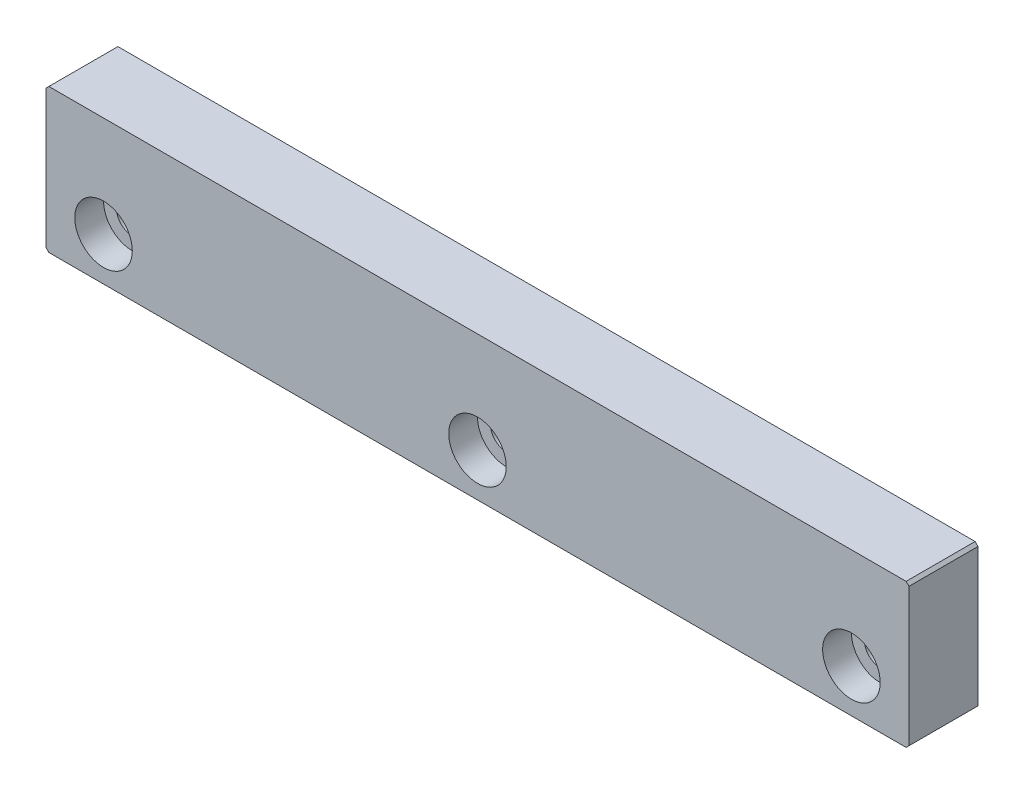
SolidWorks part; units mm, degrees
ref_plane "Front Plane" through (0, 0, 0) normal (0, 0, 1) x (1, 0, 0)
ref_plane "Top Plane" through (0, 0, 0) normal (0, 1, 0) x (1, 0, 0)
ref_plane "Right Plane" through (0, 0, 0) normal (1, 0, 0) x (0, 0, -1)
sketch "Sketch1" plane through (0, 0, 0) normal (0, 0, 1) x (1, 0, 0)
  line L1 (-75, 12.5) -> (75, 12.5)
  line L2 (-75, 12.5) -> (-75, -12.5)
  line L3 (-75, -12.5) -> (75, -12.5)
  line L4 (75, 12.5) -> (75, -12.5)
  line L5 (-75, 12.5) -> (75, -12.5) construction
  line L6 (-75, -12.5) -> (75, 12.5) construction
  point P0 (0, 0)
  dimension "D1" = 25
  dimension "D2" = 150
extrude "Boss-Extrude1" add sketch "Sketch1" along normal blind 12
hole_wizard "CBORE for M5 Hex Socket Head Cap Screw1" positions "Sketch3" profile "Sketch2" counterbore size "M5" standard "ISO" end condition through all
sketch "Sketch3" plane through (0, 0, 12) normal (0, 0, 1) x (1, 0, 0)
  line L0 (0, 12.5) -> (0, -27.2668) construction
  line L1 (75, 12.5) -> (-75, 12.5) construction
  line L3 (-75, -12.5) -> (75, -12.5) construction
  point P0 (0, -5)
  point P1 (-65, -5)
  point P3 (65, -5)
  dimension "D1" = 130
  dimension "D2" = 7.5
sketch "Sketch2" plane through (0, -5, 12) normal (1, 0, 0) x (0, -1, 0)
  line L0 (0, 0) -> (0, 12)
  line L1 (0, 12) -> (2.75, 12)
  line L3 (2.75, 12) -> (2.75, 5)
  line L4 (2.75, 5) -> (5, 5)
  line L5 (5, 5) -> (5, 0)
  line L7 (5, 0) -> (0, 0)
  line L11 (0, -6.35) -> (0, 107.95) construction
  dimension "通孔孔直径" = 5.5
  dimension "通孔孔深度" = 12
  dimension "柱形沉头孔直径" = 10
  dimension "柱形沉头孔深度" = 5
chamfer "Chamfer1" distance 0.5 angle 45 4 edges at (75, -12.5, 6) (75, 12.5, 6) (-75, 12.5, 6) (-75, -12.5, 6)
